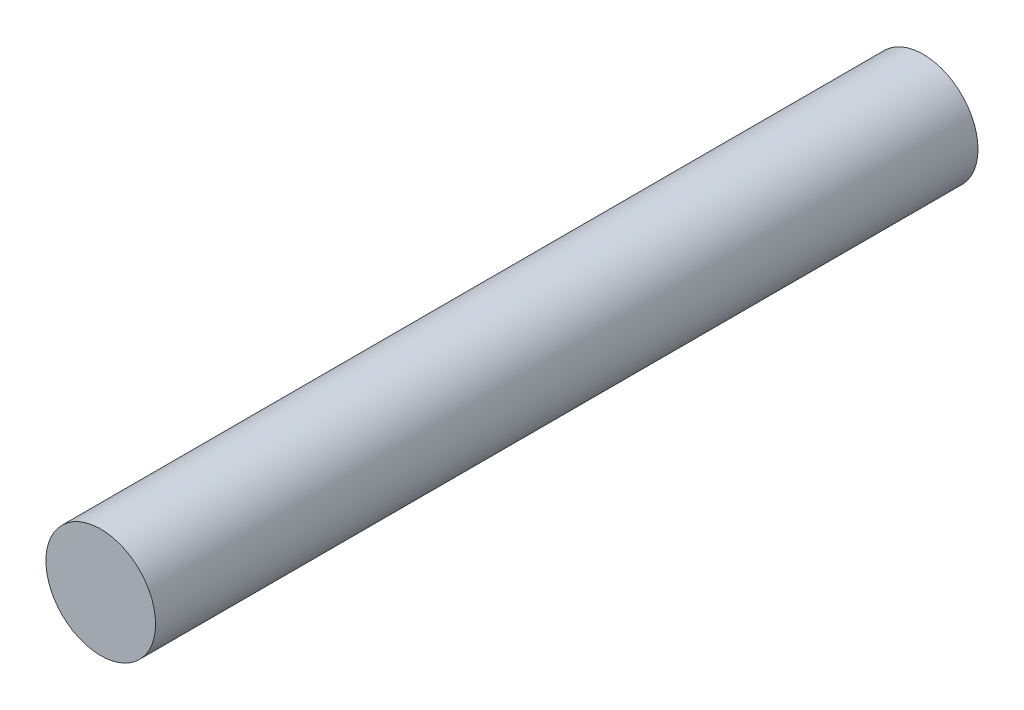
SolidWorks part; units mm, degrees
ref_plane "前视基准面" through (0, 0, 0) normal (0, 0, 1) x (1, 0, 0)
ref_plane "上视基准面" through (0, 0, 0) normal (0, 1, 0) x (1, 0, 0)
ref_plane "右视基准面" through (0, 0, 0) normal (1, 0, 0) x (0, 0, -1)
sketch "草图1" plane through (0, 0, 0) normal (0, 0, 1) x (1, 0, 0)
  circle A0 centre (0, 0) radius 10
  dimension "D1" = 20
extrude "凸台-拉伸1" add sketch "草图1" along normal mid plane 150
